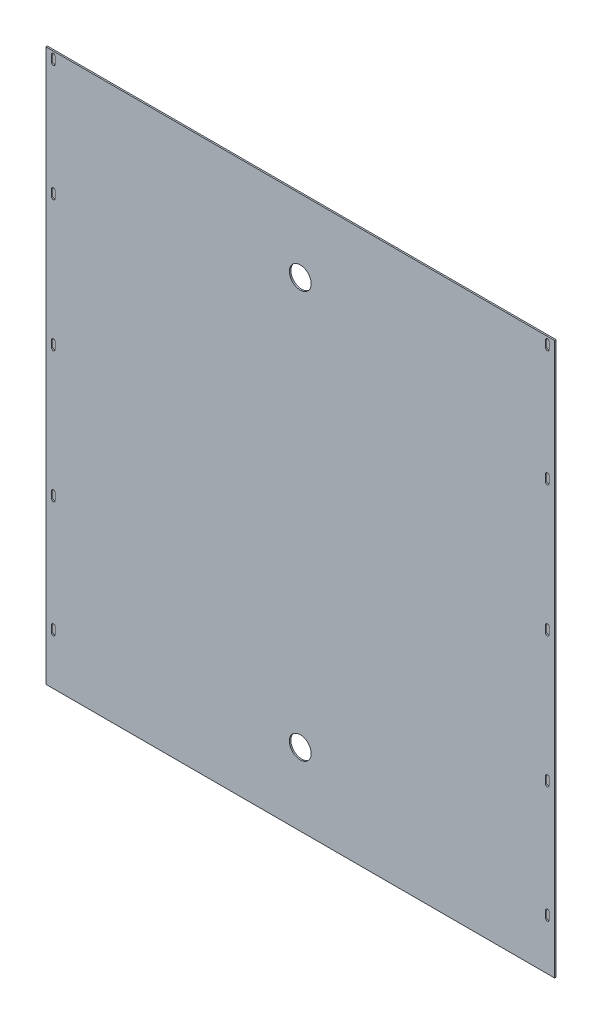
from build123d import *

# Parameters (mm, degrees)
SKETCH_1_W          = 700
SKETCH_1_H          = 760
EXTRUDE_1_DEPTH     = 2
CUT_EXTRUDE_1_DEPTH = 10
SKETCH_3_R          = 15
CUT_EXTRUDE_2_DEPTH = 10


with BuildPart() as part:
    # 草图1 → 凸台-拉伸1 (new body)
    with BuildSketch(Plane.XY):
        Rectangle(SKETCH_1_W, SKETCH_1_H)
    extrude(amount=EXTRUDE_1_DEPTH)

    # 草图2 → 切除-拉伸1 (cut)
    with BuildSketch(Plane.XY.offset(2)):
        with BuildLine():
            Line((-337.75, 375), (-337.75, 365))
            ThreePointArc((-337.75, 365), (-340, 362.75), (-342.25, 365))
            Line((-342.25, 365), (-342.25, 375))
            ThreePointArc((-342.25, 375), (-340, 377.25), (-337.75, 375))
        make_face()
        with BuildLine():
            Line((-342.25, 205), (-342.25, 215))
            ThreePointArc((-342.25, 215), (-340, 217.25), (-337.75, 215))
            Line((-337.75, 215), (-337.75, 205))
            ThreePointArc((-337.75, 205), (-340, 202.75), (-342.25, 205))
        make_face()
        with BuildLine():
            Line((-342.25, 25), (-342.25, 35))
            ThreePointArc((-342.25, 35), (-340, 37.25), (-337.75, 35))
            Line((-337.75, 35), (-337.75, 25))
            ThreePointArc((-337.75, 25), (-340, 22.75), (-342.25, 25))
        make_face()
        with BuildLine():
            Line((337.75, 375), (337.75, 365))
            ThreePointArc((337.75, 365), (340, 362.75), (342.25, 365))
            Line((342.25, 365), (342.25, 375))
            ThreePointArc((342.25, 375), (340, 377.25), (337.75, 375))
        make_face()
        with BuildLine():
            Line((342.25, 205), (342.25, 215))
            ThreePointArc((342.25, 215), (340, 217.25), (337.75, 215))
            Line((337.75, 215), (337.75, 205))
            ThreePointArc((337.75, 205), (340, 202.75), (342.25, 205))
        make_face()
        with BuildLine():
            Line((342.25, 25), (342.25, 35))
            ThreePointArc((342.25, 35), (340, 37.25), (337.75, 35))
            Line((337.75, 35), (337.75, 25))
            ThreePointArc((337.75, 25), (340, 22.75), (342.25, 25))
        make_face()
        with BuildLine():
            Line((-337.75, -315), (-337.75, -305))
            ThreePointArc((-337.75, -305), (-340, -302.75), (-342.25, -305))
            Line((-342.25, -305), (-342.25, -315))
            ThreePointArc((-342.25, -315), (-340, -317.25), (-337.75, -315))
        make_face()
        with BuildLine():
            Line((-337.75, -155), (-337.75, -145))
            ThreePointArc((-337.75, -145), (-340, -142.75), (-342.25, -145))
            Line((-342.25, -145), (-342.25, -155))
            ThreePointArc((-342.25, -155), (-340, -157.25), (-337.75, -155))
        make_face()
        with BuildLine():
            Line((337.75, -315), (337.75, -305))
            ThreePointArc((337.75, -305), (340, -302.75), (342.25, -305))
            Line((342.25, -305), (342.25, -315))
            ThreePointArc((342.25, -315), (340, -317.25), (337.75, -315))
        make_face()
        with BuildLine():
            Line((342.25, -145), (342.25, -155))
            ThreePointArc((342.25, -155), (340, -157.25), (337.75, -155))
            Line((337.75, -155), (337.75, -145))
            ThreePointArc((337.75, -145), (340, -142.75), (342.25, -145))
        make_face()
    extrude(amount=-CUT_EXTRUDE_1_DEPTH, mode=Mode.SUBTRACT)

    # 草图3 → 切除-拉伸2 (cut)
    with BuildSketch(Plane.XY.offset(2)):
        with Locations((0, -280)):
            Circle(SKETCH_3_R)
        with Locations((0, 280)):
            Circle(SKETCH_3_R)
    extrude(amount=-CUT_EXTRUDE_2_DEPTH, mode=Mode.SUBTRACT)


solid = part.part
